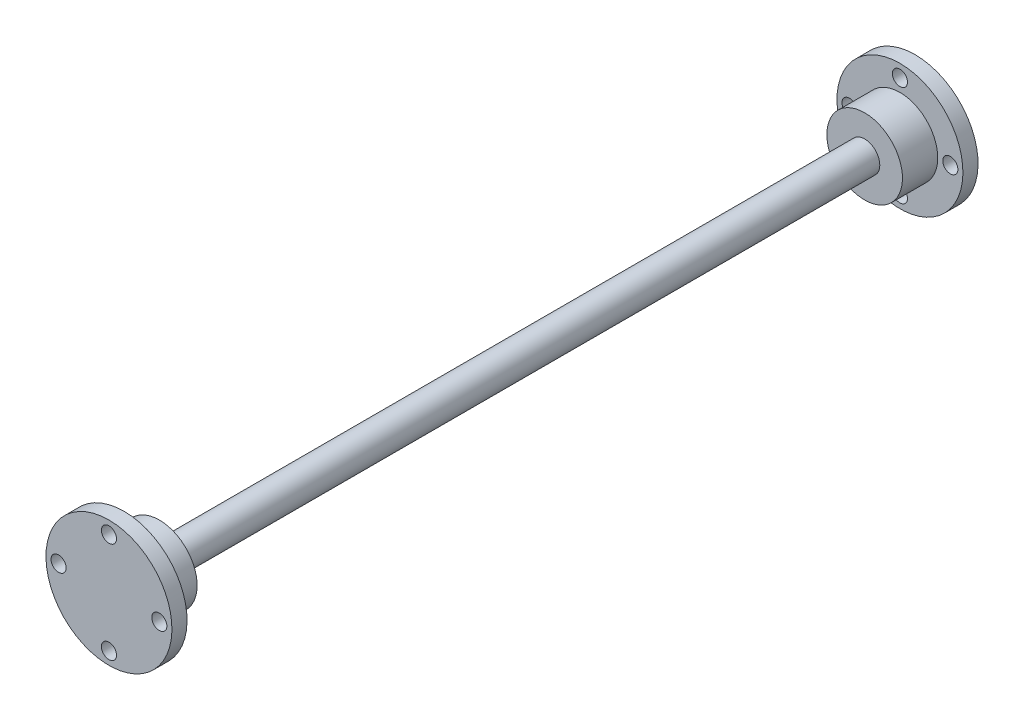
SolidWorks part; units mm, degrees
other "Annotation1"
sketch "草图6" plane through (12.5, 12.5, 70) normal (0.1491, 0.0743, 0.986) x (0.5255, -0.8507, -0.0154)
ref_plane "Front Plane" through (0, 0, 0) normal (0, 0, 1) x (1, 0, 0)
ref_plane "Top Plane" through (0, 0, 0) normal (0, 1, 0) x (1, 0, 0)
ref_plane "Right Plane" through (0, 0, 0) normal (1, 0, 0) x (0, 0, -1)
other "Configuration Table"
sketch "Sketch4" plane through (0, 0, 0) normal (1, 0, 0) x (0, 0, -1)
  line L0 (0, 41.6509) -> (0, 0) construction
  line L1 (0, 0) -> (-80, 0) construction
  line L2 (-80, 0) -> (-80, 12.5)
  line L3 (-80, 12.5) -> (-77, 12.5)
  line L4 (-77, 12.5) -> (-77, 7.5)
  line L5 (-77, 7.5) -> (-70, 7.5)
  line L6 (-70, 7.5) -> (-70, 3)
  line L7 (-70, 3) -> (0, 3)
  line L8 (0, 3) -> (0, 0)
  line L9 (0, 0) -> (-80, 0)
  dimension "D1" = 80
  dimension "D2" = 25
  dimension "D3" = 15
  dimension "D4" = 6
  dimension "D5" = 3
  dimension "D6" = 7
revolve "Revolve2" add sketch "Sketch4" angle 360 about L9
ref_plane "Plane1" through (0, 0, 0) normal (0, 0, -1) x (-1, 0, 0)
mirror "Mirror1" about plane through (0, 0, 0) normal (0, 0, -1) of "Revolve2"
sketch "Sketch5" plane through (0, 0, -80) normal (0, 0, -1) x (-1, 0, 0)
  line L0 (0, 0) -> (7.5, 0) construction
  line L1 (0, 0) -> (0, 7.5) construction
  circle A0 centre (0, 0) radius 7.5 construction
  circle A1 centre (10, 0) radius 1.5
  circle A2 centre (0, -10) radius 1.5
  circle A3 centre (-10, 0) radius 1.5
  circle A4 centre (0, 10) radius 1.5
  point P16 (0, 0)
  dimension "D1" = 15
  dimension "D2" = 3
  dimension "D3" = 10
  dimension "D4" = 4
extrude "Cut-Extrude4" cut sketch "Sketch5" against normal blind 164
